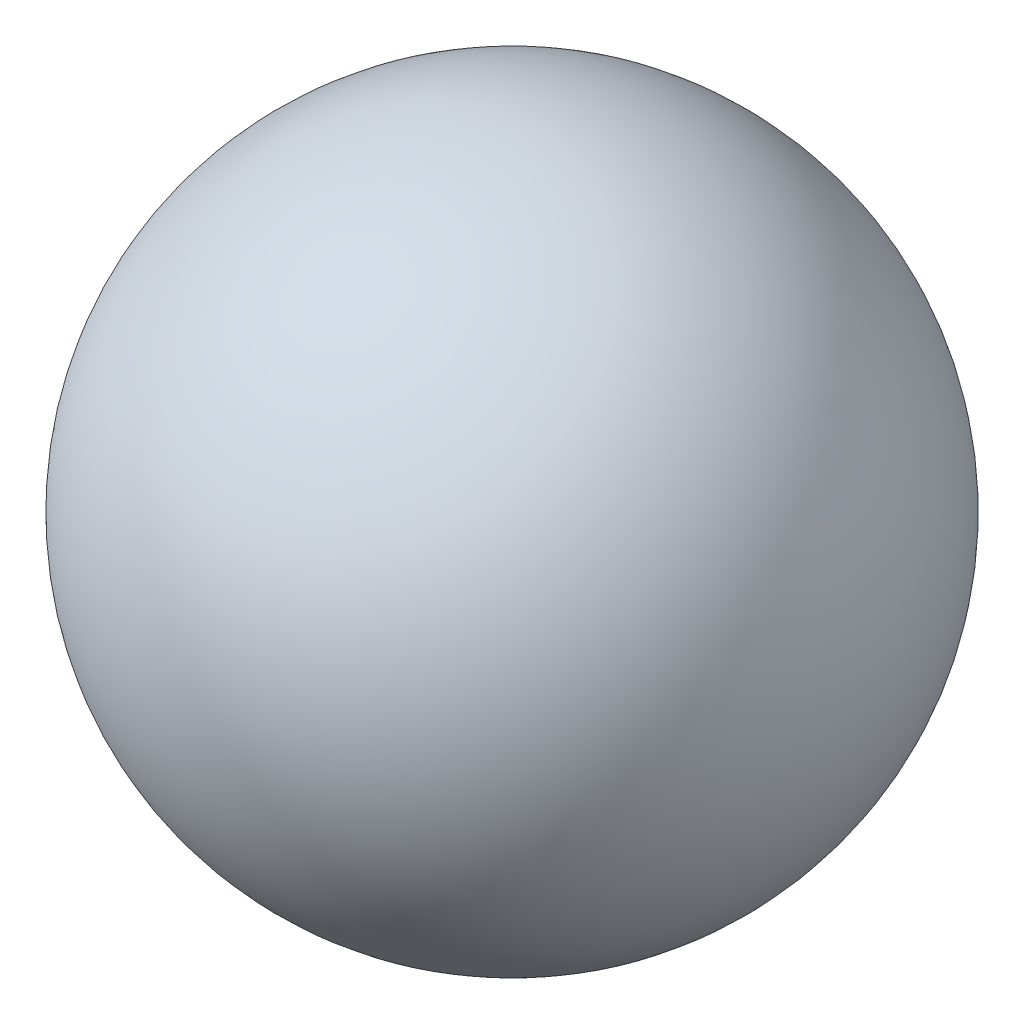
from build123d import *


with BuildPart() as part:
    # 草图1 → 旋转1 (revolve)
    with BuildSketch(Plane.XY):
        with BuildLine():
            Line((0, 50), (0, -50))
            ThreePointArc((0, -50), (50, 0), (0, 50))
        make_face()
    revolve(axis=Axis((0, 50, 0), (0, -1, 0)))


solid = part.part
